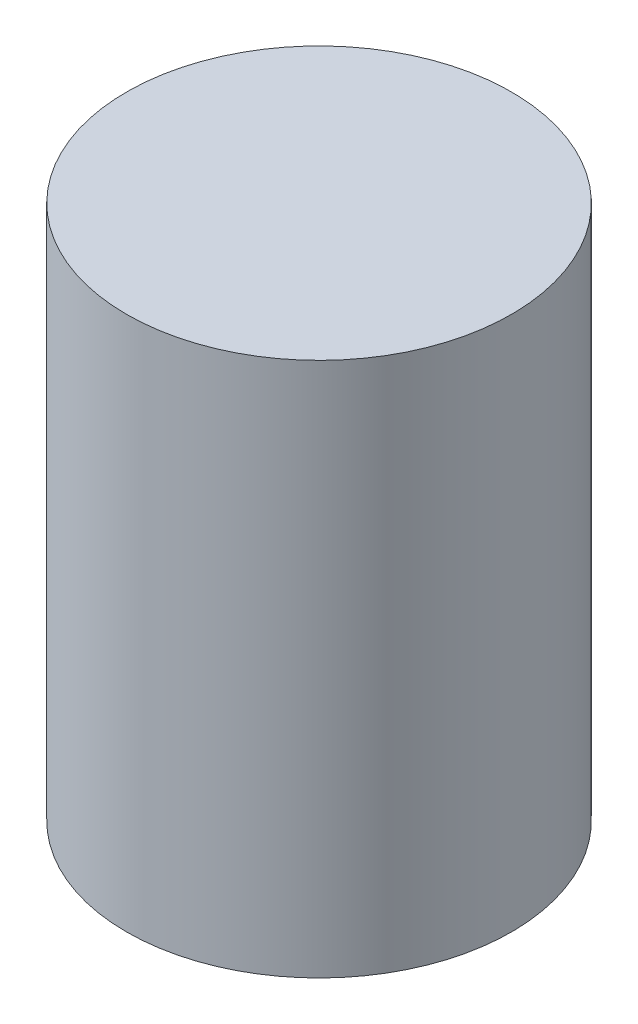
from build123d import *

# Parameters (mm, degrees)
SKETCH_1_R      = 9
EXTRUDE_1_DEPTH = 12.5


with BuildPart() as part:
    # 草图1 → 凸台-拉伸1 (new, symmetric)
    with BuildSketch(Plane(origin=(0, 0, 0), x_dir=(1, 0, 0), z_dir=(0, 1, 0))):
        with Locations(Location((0, 0, 0), (0, 0, 270))):
            Circle(SKETCH_1_R)
    extrude(amount=EXTRUDE_1_DEPTH, both=True)


solid = part.part
